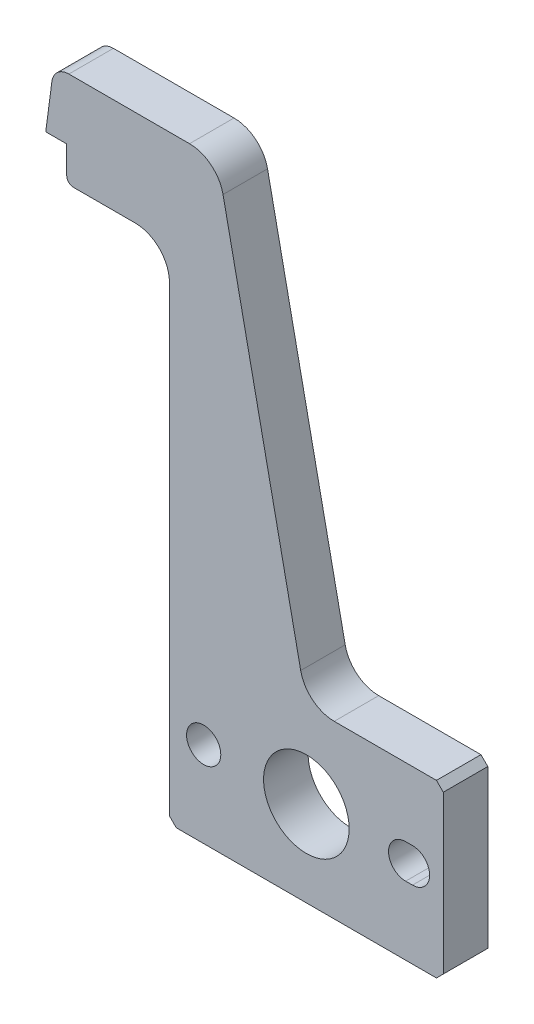
SolidWorks part; units mm, degrees
ref_plane "Front Plane" through (0, 0, 0) normal (0, 0, 1) x (1, 0, 0)
ref_plane "Top Plane" through (0, 0, 0) normal (0, 1, 0) x (1, 0, 0)
ref_plane "Right Plane" through (0, 0, 0) normal (1, 0, 0) x (0, 0, -1)
sketch "Sketch1" plane through (0, 0, 0) normal (0, 0, 1) x (1, 0, 0)
  line L1 (-5.8, 8.75) -> (5.8, 8.75)
  line L2 (-5.8, 8.75) -> (-5.8, -8.75)
  line L3 (-5.8, -8.75) -> (5.8, -8.75)
  line L4 (5.8, 8.75) -> (5.8, -8.75)
  line L5 (-5.8, 8.75) -> (5.8, -8.75) construction
  line L6 (-5.8, -8.75) -> (5.8, 8.75) construction
  point P0 (0, 0)
  dimension "D1" = 11.6
  dimension "D2" = 17.5
extrude "Boss-Extrude1" add sketch "Sketch1" along normal mid plane 1.3
sketch "Sketch2" plane through (0, 0, 0.65) normal (0, 0, 1) x (1, 0, 0)
  line L0 (4.7, -6.25) -> (4.9, -6.25) construction
  line L1 (4.7, -5.75) -> (4.9, -5.75)
  line L2 (4.7, -6.75) -> (4.9, -6.75)
  line L3 (-5.8, -8.75) -> (5.8, -8.75) construction
  line L4 (5.8, -8.75) -> (5.8, 8.75) construction
  circle A0 centre (1.8, -6.25) radius 1.25
  circle A1 centre (-1.2, -6.25) radius 0.5
  arc A2 (4.7, -5.75) -> (4.7, -6.75) centre (4.7, -6.25) ccw
  arc A3 (4.9, -6.75) -> (4.9, -5.75) centre (4.9, -6.25) ccw
  point P6 (4.8, -6.25)
  dimension "D1" = 1
  dimension "D2" = 2.5
  dimension "D3" = 1
  dimension "D4" = 0.2
  dimension "D5" = 6
  dimension "D6" = 2.5
  dimension "D7" = 4
  dimension "D8" = 3
extrude "Cut-Extrude1" cut sketch "Sketch2" against normal through all
sketch "Sketch3" plane through (0, 0, 0.65) normal (0, 0, 1) x (1, 0, 0)
  line L0 (5.8, -8.75) -> (5.8, 8.75) construction
  line L1 (-5.8, -8.75) -> (-2.2, -8.75)
  line L2 (-5.8, -8.75) -> (-5.8, 5.95)
  line L3 (-5.8, 5.95) -> (-2.2, 5.95)
  line L4 (-2.2, -8.75) -> (-2.2, 5.95)
  line L5 (5.8, 8.75) -> (-5.8, 8.75) construction
  line L6 (5.8, -3.75) -> (1.8, -3.75)
  line L7 (1.8, -3.75) -> (-0.8, 8.75)
  line L8 (-0.8, 8.75) -> (5.8, 8.75)
  line L9 (5.8, 8.75) -> (5.8, -3.75)
  line L10 (-5.8, -8.75) -> (5.8, -8.75) construction
  line L11 (-5.8, 8.75) -> (-5.8, -8.75) construction
  dimension "D1" = 8
  dimension "D2" = 2.8
  dimension "D3" = 5
  dimension "D4" = 5
  dimension "D5" = 4
extrude "Cut-Extrude2" cut sketch "Sketch3" against normal through all
sketch "Sketch4" plane through (0, 0, 0.65) normal (0, 0, 1) x (1, 0, 0)
  line L1 (-5.8, 5.95) -> (-5.2, 5.95)
  line L2 (-5.8, 5.95) -> (-5.8, 6.95)
  line L3 (-5.8, 6.95) -> (-5.2, 6.95)
  line L4 (-5.2, 5.95) -> (-5.2, 6.95)
  dimension "D1" = 1
  dimension "D2" = 0.6
extrude "Cut-Extrude3" cut sketch "Sketch4" against normal through all
fillet "Fillet2" radius 0.2 1 edges at (-5.2, 5.95, 0)
sketch "Sketch5" plane through (0, 0, 0.65) normal (0, 0, 1) x (1, 0, 0)
  line L0 (-5.8, 7.05) -> (-5.5762, 8.75)
  line L1 (-0.8, 8.75) -> (-5.8, 8.75) construction
  line L2 (-5.5762, 8.75) -> (-5.8, 8.75)
  line L3 (-5.8, 8.75) -> (-5.8, 7.05)
  line L4 (-5.8, 8.75) -> (-5.8, 6.95) construction
  line L5 (-5.2, 6.95) -> (-5.8, 6.95) construction
  dimension "D1" = 7.5
  dimension "D2" = 0.1
extrude "Cut-Extrude4" cut sketch "Sketch5" against normal through all
fillet "Fillet3" radius 1 3 edges at (-0.8, 8.75, 0) (-2.2, 5.95, 0) (1.8, -3.75, 0)
chamfer "Chamfer1" distance 0.2 angle 45 3 edges at (5.8, -3.75, 0) (5.8, -8.75, 0) (-2.2, -8.75, 0)
fillet "Fillet4" radius 0.5 1 edges at (-5.5762, 8.75, 0)
